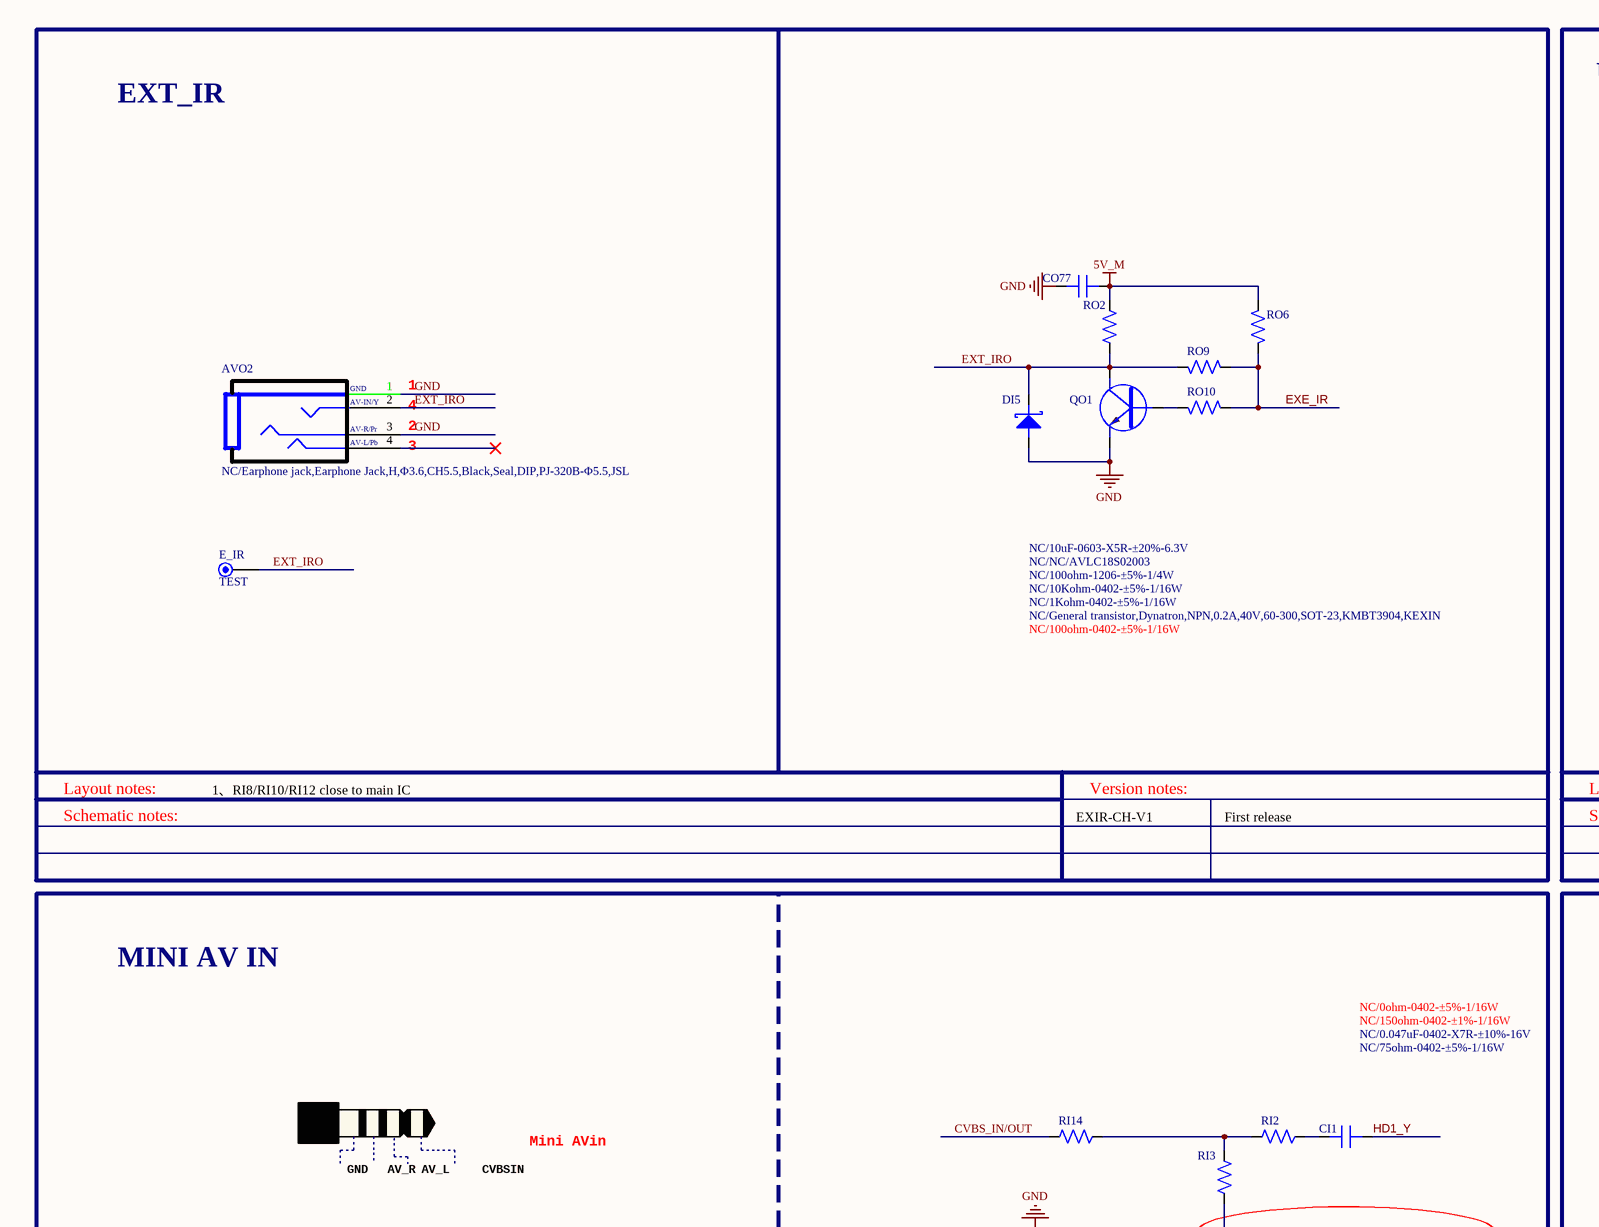
[diagram p0: MISC86383-13.SchDoc, top left]
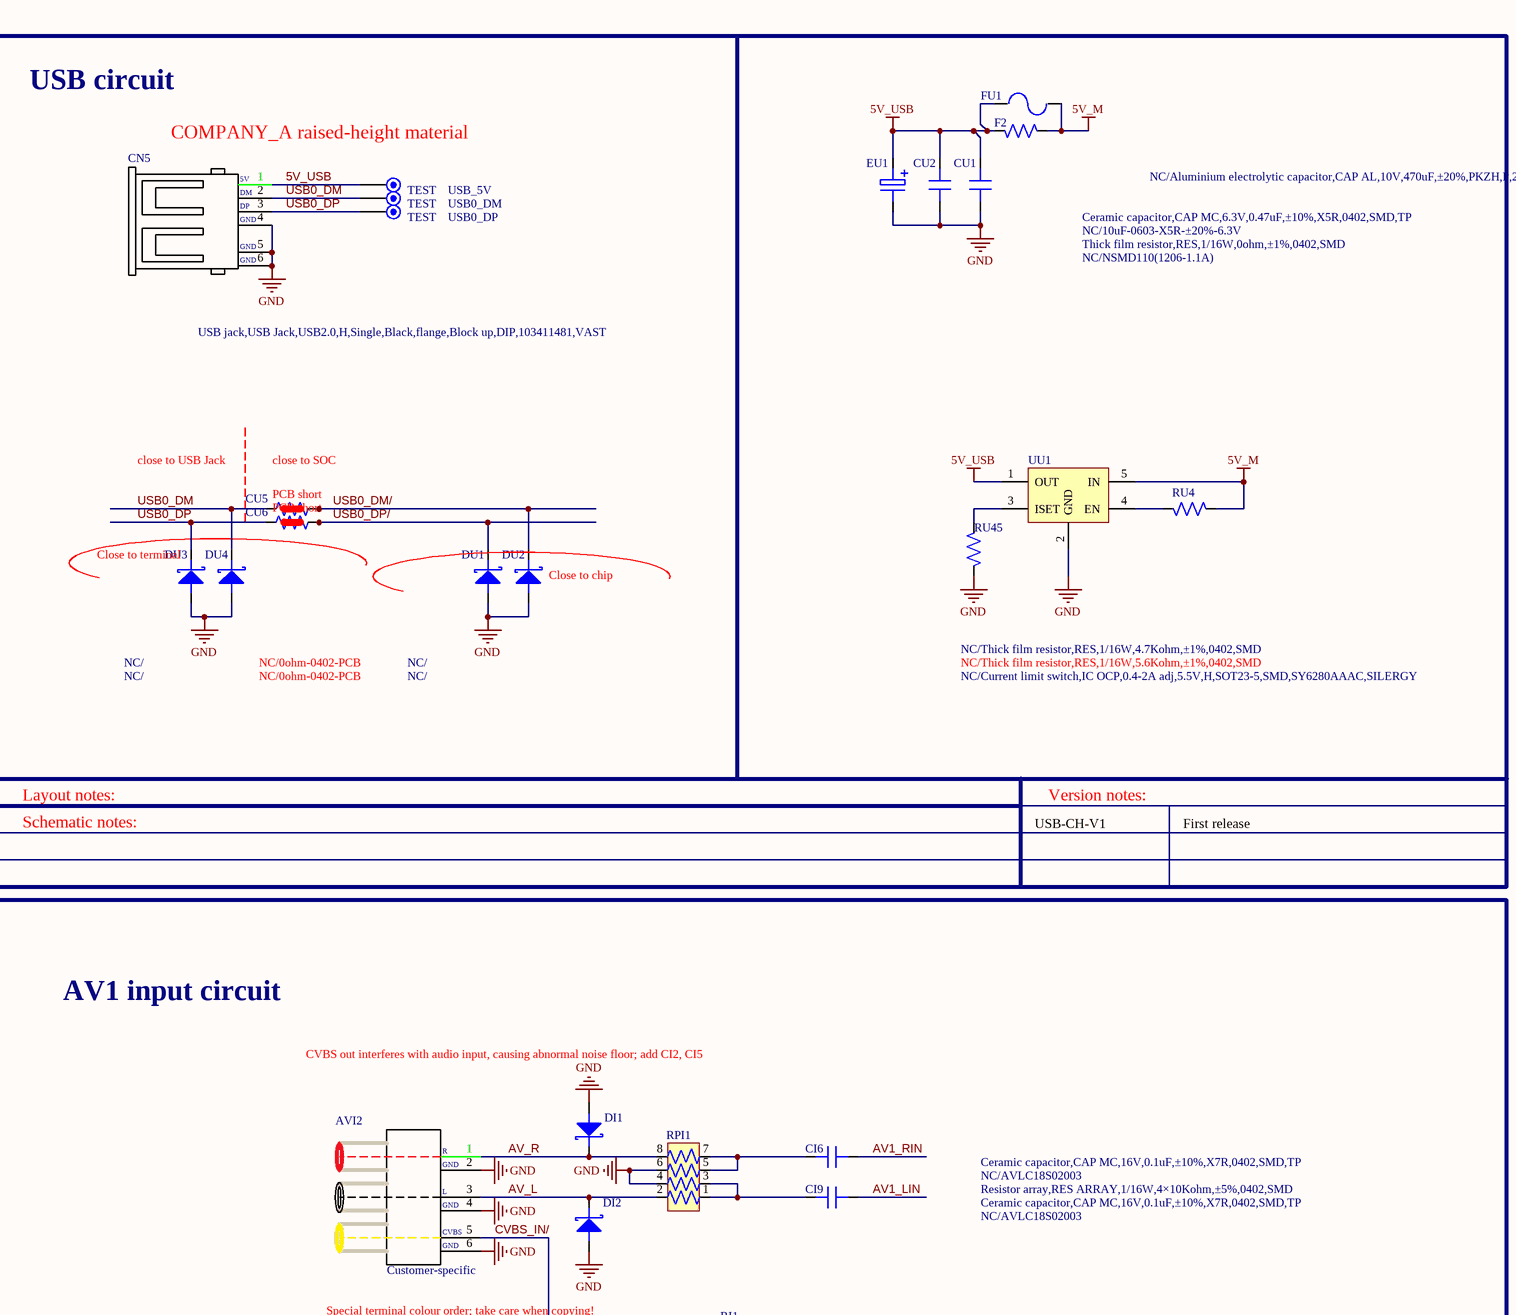
[diagram p1: MISC86383-13.SchDoc, top right]
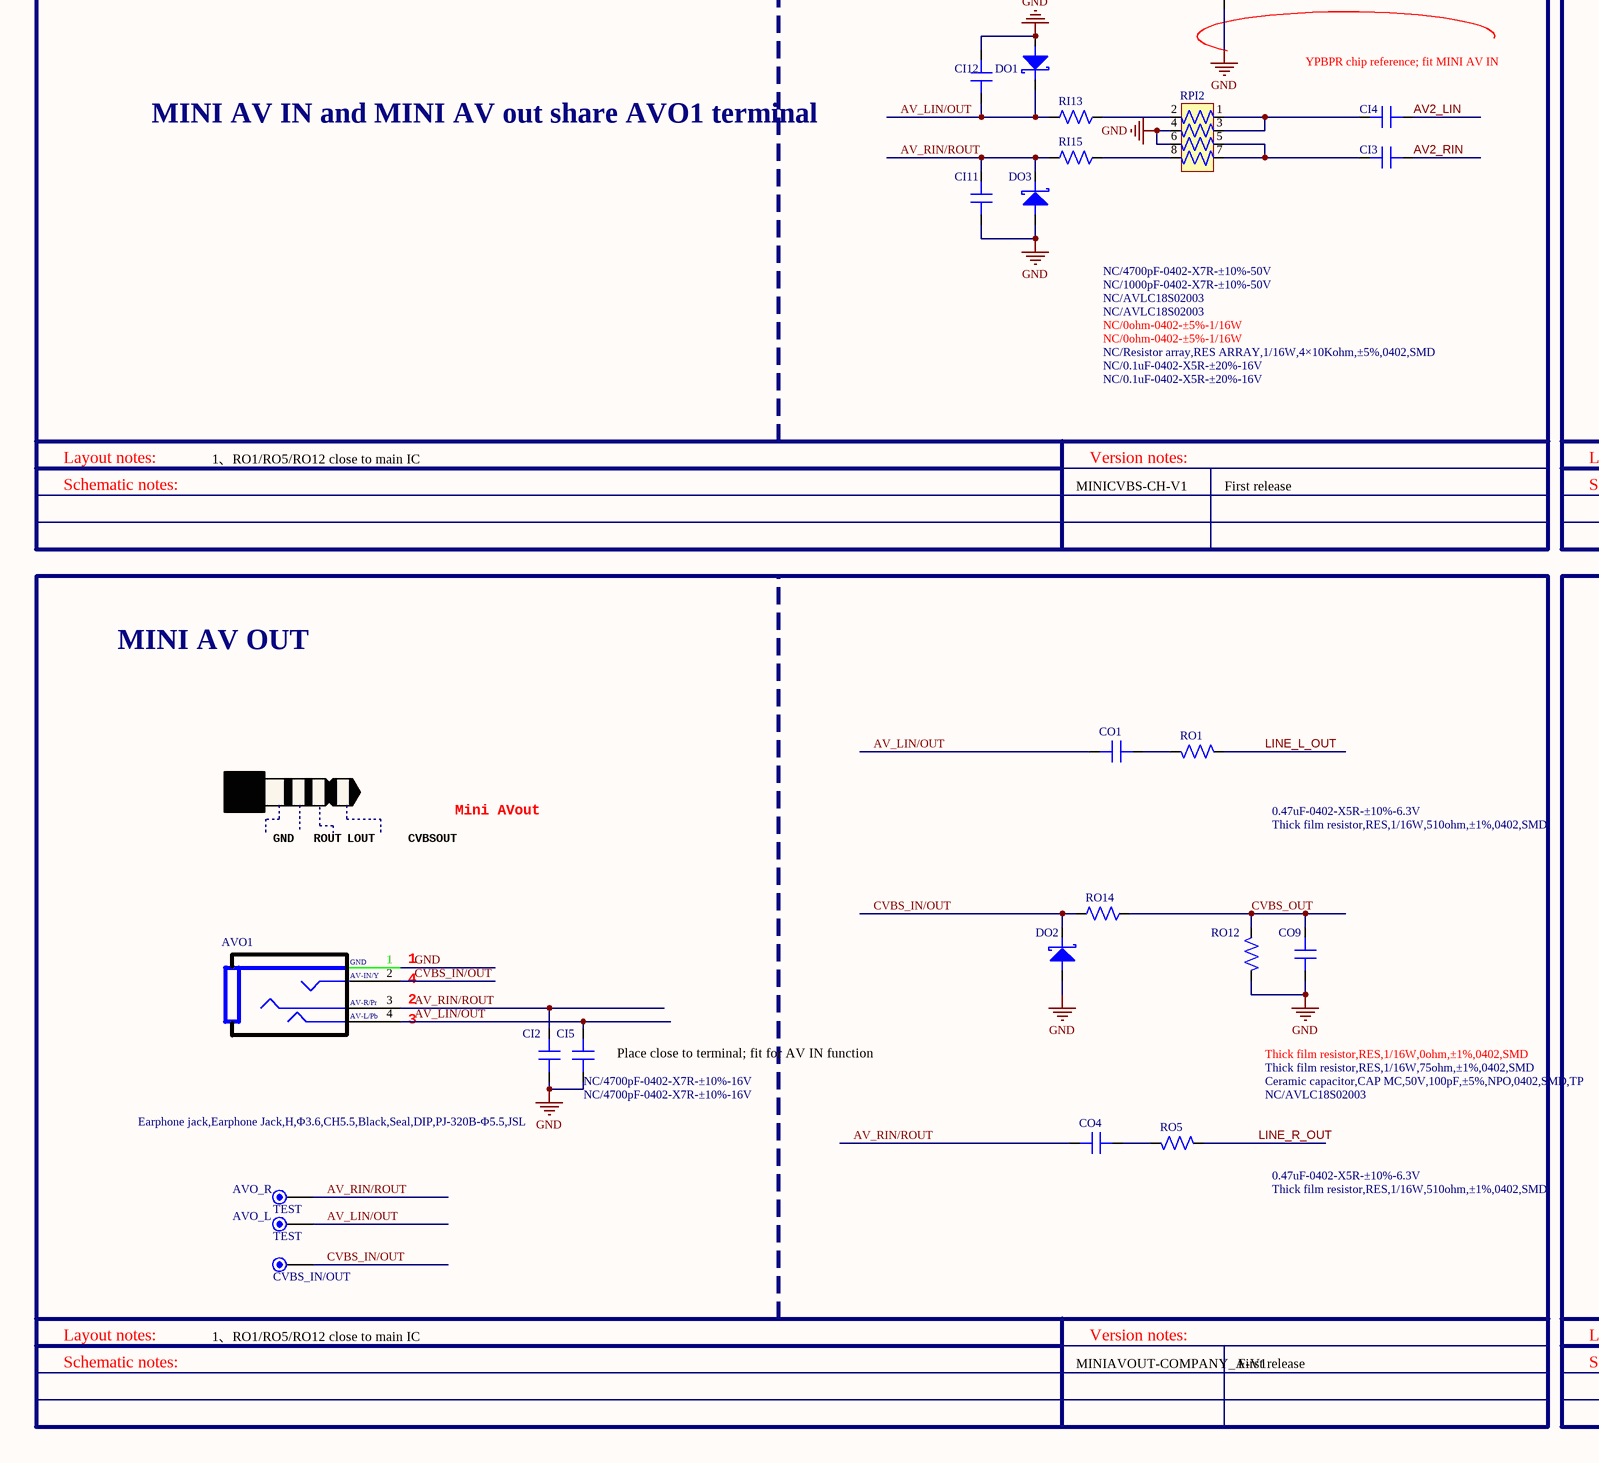
[diagram p2: MISC86383-13.SchDoc, bottom left]
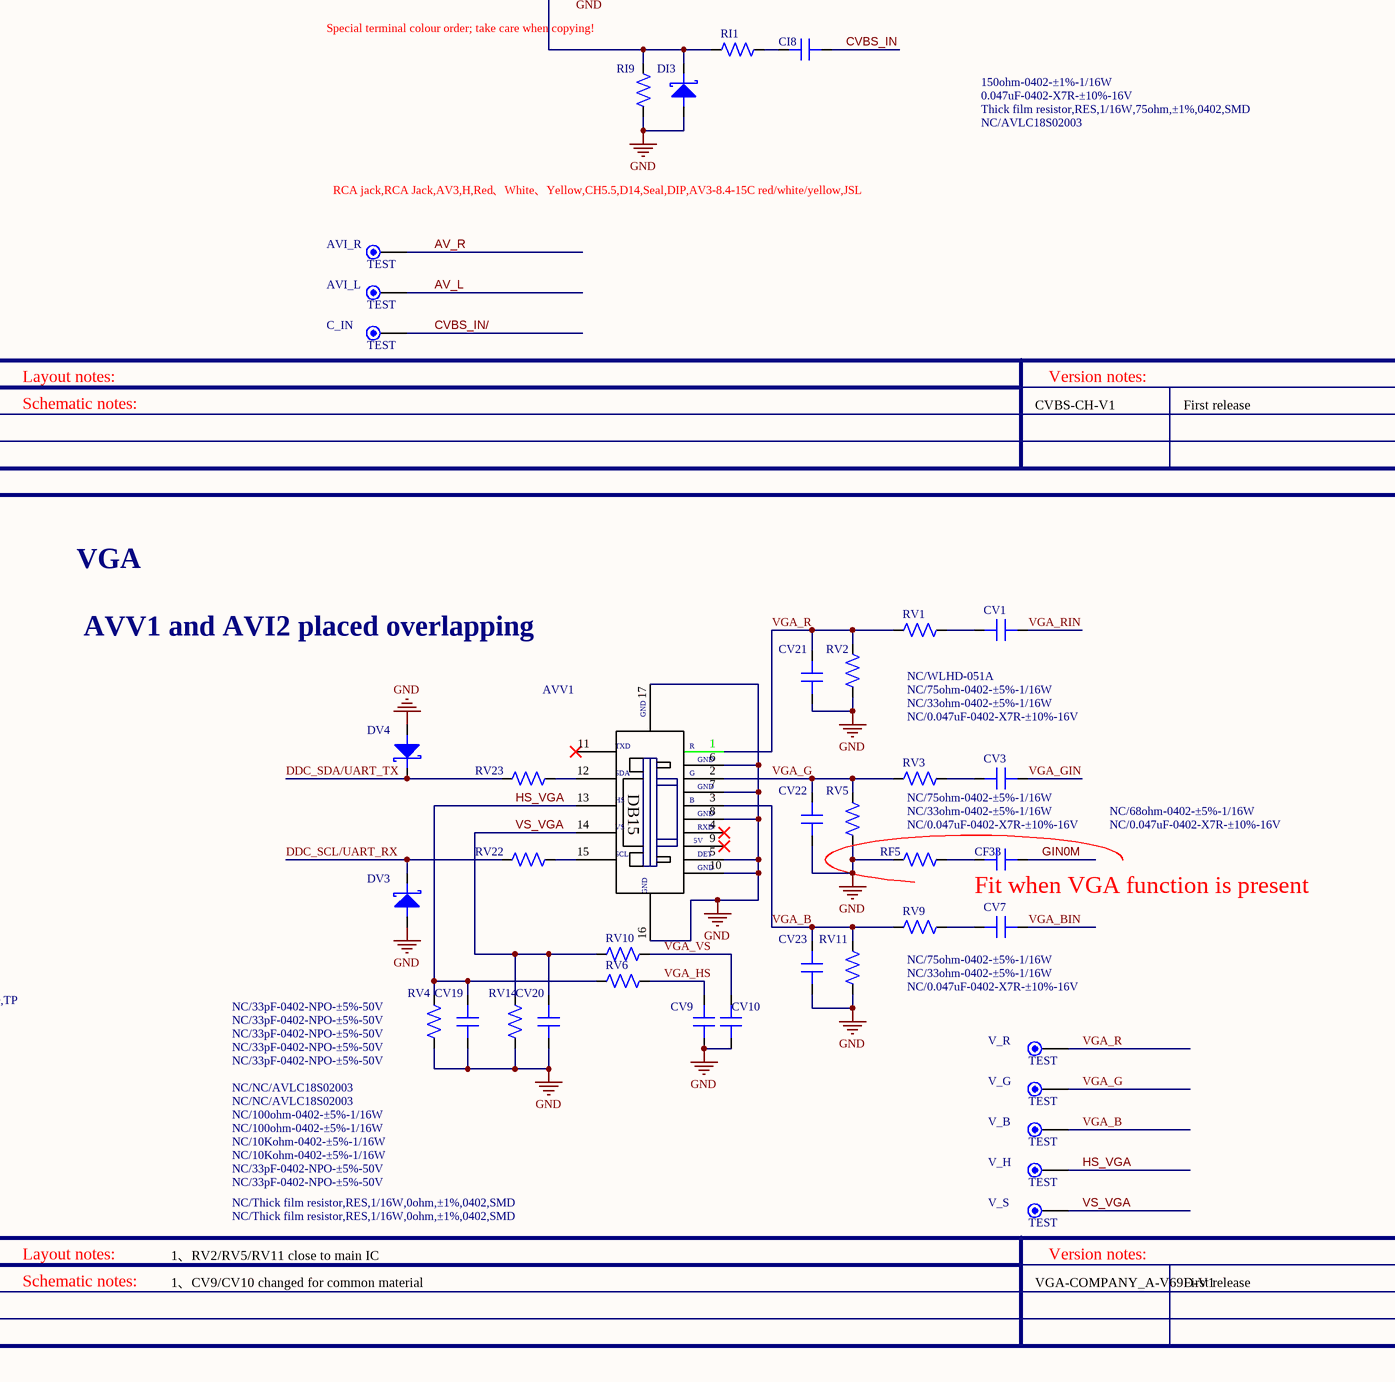
[diagram p3: MISC86383-13.SchDoc, bottom right]
# Altium project MISC86383-33.PrjPCB (part 3 of 8)

## Sheet MISC86383-13.SchDoc
size 609 x 546 mm

### Parts
AVI2  RCA jack,RCA Jack,AV3,H,Red、White、Yellow,CH5.5,D14,Seal,DIP,AV3-8.4-15C red/white/yellow,JSL  [AV3-H14-15]
AVI_L  TEST  [TP]
AVI_R  TEST  [TP]
AVO1  Earphone jack,Earphone Jack,H,Φ3.6,CH5.5,Black,Seal,DIP,PJ-320B-Φ5.5,JSL  [PHONE-HD-43]
AVO2  NC/Earphone jack,Earphone Jack,H,Φ3.6,CH5.5,Black,Seal,DIP,PJ-320B-Φ5.5,JSL  [PHONE-HD-43]
AVO_L  TEST  [TP]
AVO_R  TEST  [TP]
AVV1  NC/WLHD-051A  [DB15-HF-1]
C_IN  TEST  [TP]
CF33  NC/0.047uF-0402-X7R-±10%-16V  [C0402]
CI1  NC/0.047uF-0402-X7R-±10%-16V  [C0402]
CI2  NC/4700pF-0402-X7R-±10%-16V  [C0402]
CI3  NC/0.1uF-0402-X5R-±20%-16V  [C0402]
CI4  NC/0.1uF-0402-X5R-±20%-16V  [C0402]
CI5  NC/4700pF-0402-X7R-±10%-16V  [C0402]
CI6  Ceramic capacitor,CAP MC,16V,0.1uF,±10%,X7R,0402,SMD,TP  [C0402]
CI8  0.047uF-0402-X7R-±10%-16V  [C0402]
CI9  Ceramic capacitor,CAP MC,16V,0.1uF,±10%,X7R,0402,SMD,TP  [C0402]
CI11  NC/1000pF-0402-X7R-±10%-50V  [C0402]
CI12  NC/4700pF-0402-X7R-±10%-50V  [C0402]
CN5  USB jack,USB Jack,USB2.0,H,Single,Black,flange,Block up,DIP,103411481,VAST  [USB-HD-30]
CO1  0.47uF-0402-X5R-±10%-6.3V  [C0402]
CO4  0.47uF-0402-X5R-±10%-6.3V  [C0402]
CO9  Ceramic capacitor,CAP MC,50V,100pF,±5%,NPO,0402,SMD,TP  [C0402]
CO77  NC/10uF-0603-X5R-±20%-6.3V  [C0603]
CU1  NC/10uF-0603-X5R-±20%-6.3V  [C0603]
CU2  Ceramic capacitor,CAP MC,6.3V,0.47uF,±10%,X5R,0402,SMD,TP  [C0402]
CU5  NC/0ohm-0402-PCB  [R0402SC]
CU6  NC/0ohm-0402-PCB  [R0402SC]
CV1  NC/0.047uF-0402-X7R-±10%-16V  [C0402]
CV3  NC/0.047uF-0402-X7R-±10%-16V  [C0402]
CV7  NC/0.047uF-0402-X7R-±10%-16V  [C0402]
CV9  NC/33pF-0402-NPO-±5%-50V  [C0402]
CV10  NC/33pF-0402-NPO-±5%-50V  [C0402]
CV19  NC/33pF-0402-NPO-±5%-50V  [C0402]
CV20  NC/33pF-0402-NPO-±5%-50V  [C0402]
CV21  NC/33pF-0402-NPO-±5%-50V  [C0402]
CV22  NC/33pF-0402-NPO-±5%-50V  [C0402]
CV23  NC/33pF-0402-NPO-±5%-50V  [C0402]
CVBS_IN/OUT  TEST  [TP]  (value not drawn)
DI1  NC/AVLC18S02003  [DIODE-S0402]
DI2  NC/AVLC18S02003  [DIODE-S0402]
DI3  NC/AVLC18S02003  [DIODE-S0402]
DI5  NC/NC/AVLC18S02003  [DIODE-S0402]
DO1  NC/AVLC18S02003  [DIODE-S0402]
DO2  NC/AVLC18S02003  [DIODE-S0402]
DO3  NC/AVLC18S02003  [DIODE-S0402]
DU1  NC/  [DIODE-S0402]
DU2  NC/  [DIODE-S0402]
DU3  NC/  [DIODE-S0402]
DU4  NC/  [DIODE-S0402]
DV3  NC/NC/AVLC18S02003  [DIODE-S0402]
DV4  NC/NC/AVLC18S02003  [DIODE-S0402]
E_IR  TEST  [TP]
EU1  NC/Aluminium electrolytic capacitor,CAP AL,10V,470uF,±20%,PKZH,P,2.5mm,6.3×11,DIP,TP,Koshin  [EC(6.3*11)-V-2.5]
F2  Thick film resistor,RES,1/16W,0ohm,±1%,0402,SMD  [R0402]
FU1  NC/NSMD110(1206-1.1A)  [FUSE1.1A-S]
QO1  NC/General transistor,Dynatron,NPN,0.2A,40V,60-300,SOT-23,KMBT3904,KEXIN  [SOT-23]
RF5  NC/68ohm-0402-±5%-1/16W  [R0402]
RI1  150ohm-0402-±1%-1/16W  [R0402]
RI2  NC/150ohm-0402-±1%-1/16W  [R0402]
RI3  NC/75ohm-0402-±5%-1/16W  [R0402]
RI9  Thick film resistor,RES,1/16W,75ohm,±1%,0402,SMD  [R0402]
RI13  NC/0ohm-0402-±5%-1/16W  [R0402]
RI14  NC/0ohm-0402-±5%-1/16W  [R0402]
RI15  NC/0ohm-0402-±5%-1/16W  [R0402]
RO1  Thick film resistor,RES,1/16W,510ohm,±1%,0402,SMD  [R0402]
RO2  NC/100ohm-1206-±5%-1/4W  [R1206]
RO5  Thick film resistor,RES,1/16W,510ohm,±1%,0402,SMD  [R0402]
RO6  NC/10Kohm-0402-±5%-1/16W  [R0402]
RO9  NC/100ohm-0402-±5%-1/16W  [R0402]
RO10  NC/1Kohm-0402-±5%-1/16W  [R0402]
RO12  Thick film resistor,RES,1/16W,75ohm,±1%,0402,SMD  [R0402]
RO14  Thick film resistor,RES,1/16W,0ohm,±1%,0402,SMD  [R0402]
RPI1  Resistor array,RES ARRAY,1/16W,4×10Kohm,±5%,0402,SMD  [RA0402]
RPI2  NC/Resistor array,RES ARRAY,1/16W,4×10Kohm,±5%,0402,SMD  [RA0402]
RU4  NC/Thick film resistor,RES,1/16W,4.7Kohm,±1%,0402,SMD  [R0402]
RU45  NC/Thick film resistor,RES,1/16W,5.6Kohm,±1%,0402,SMD  [R0402]
RV1  NC/33ohm-0402-±5%-1/16W  [R0402]
RV2  NC/75ohm-0402-±5%-1/16W  [R0402]
RV3  NC/33ohm-0402-±5%-1/16W  [R0402]
RV4  NC/10Kohm-0402-±5%-1/16W  [R0402]
RV5  NC/75ohm-0402-±5%-1/16W  [R0402]
RV6  NC/100ohm-0402-±5%-1/16W  [R0402]
RV9  NC/33ohm-0402-±5%-1/16W  [R0402]
RV10  NC/100ohm-0402-±5%-1/16W  [R0402]
RV11  NC/75ohm-0402-±5%-1/16W  [R0402]
RV14  NC/10Kohm-0402-±5%-1/16W  [R0402]
RV22  NC/Thick film resistor,RES,1/16W,0ohm,±1%,0402,SMD  [R0402]
RV23  NC/Thick film resistor,RES,1/16W,0ohm,±1%,0402,SMD  [R0402]
USB0_DM  TEST  [TP]
USB0_DP  TEST  [TP]
USB_5V  TEST  [TP]
UU1  NC/Current limit switch,IC OCP,0.4-2A adj,5.5V,H,SOT23-5,SMD,SY6280AAAC,SILERGY  [SOP23-5-1]
V_B  TEST  [TP]
V_G  TEST  [TP]
V_H  TEST  [TP]
V_R  TEST  [TP]
V_S  TEST  [TP]

### Blocks framed on the sheet
EXT_IR: AVO2 CO77 DI5 E_IR QO1 RO2 RO6 RO9 RO10
USB circuit: CN5 CU1 CU2 CU5 CU6 DU1-DU4 EU1 F2 FU1 RU4 RU45 USB0_DM USB0_DP USB_5V UU1
AV1 input circuit: AVI2 AVI_L AVI_R C_IN CI6 CI8 CI9 DI1-DI3 RI1 RI9 RPI1
MINI AV OUT: AVO1 AVO_L AVO_R CI2 CI5 CO1 CO4 CO9 CVBS_IN/OUT DO2 RO1 RO5 RO12 RO14

### Nets
5V_M: CO77.1 F2.1 FU1.2 RO2.2 RO6.1 RU4.2 UU1.5(IN)
5V_USB: CN5.1 CU1.2 CU2.1 EU1.1 F2.2 FU1.1 USB_5V.1 UU1.1(OUT)
GND: AVI2.2(GND) AVI2.4(GND) AVI2.6(GND) AVO1.1 AVO2.1 AVO2.3 AVV1.5 AVV1.6(GND) AVV1.7(GND) AVV1.8(GND) AVV1.10(GND) AVV1.16(Shell) AVV1.17(Shell) CI2.1 CI5.1 CI11.2 CI12.2 CN5.4 CN5.5 CN5.6 CO9.1 CO77.2 CU1.1 CU2.2 CV9.1 CV10.1 CV19.1 CV20.1 CV21.1 CV22.1 CV23.1 DI1.A DI2.A DI3.A DI5.A DO1.A DO2.A DO3.A DU1.A DU2.A DU3.A DU4.A DV3.A DV4.A EU1.2 QO1.E RF5.2 RI3.1 RI9.1 RO12.2 RPI1.4 RPI1.6 RPI2.4 RPI2.6 RU45.2 RV2.1 RV4.2 RV5.1 RV11.1 RV14.2 UU1.2(GND)
AV1_LIN: CI9.1
AV1_RIN: CI6.1
AV2_LIN: CI4.1
AV2_RIN: CI3.1
AV_L: AVI2.3(Rin) AVI_L.1 DI2.K RPI1.2
AV_LIN/OUT: AVO1.4 AVO_L.1 CI5.2 CI12.1 CO1.1 DO1.K RI13.1
AV_R: AVI2.1(Lin) AVI_R.1 DI1.K RPI1.8
AV_RIN/ROUT: AVO1.3 AVO_R.1 CI2.2 CI11.1 CO4.1 DO3.K RI15.1
CVBS_IN: CI8.1
CVBS_IN/: AVI2.5(CVBS) C_IN.1 DI3.K RI1.1 RI9.2
CVBS_IN/OUT: AVO1.2 CVBS_IN/OUT.1 DO2.K RI14.1 RO14.1
CVBS_OUT: CO9.2 RO12.1 RO14.2
DDC_SCL/UART_RX: DV3.K RV22.1
DDC_SDA/UART_TX: DV4.K RV23.1
EXE_IR: RO6.2 RO9.2 RO10.2
EXT_IRO: AVO2.2 DI5.K E_IR.1 QO1.C RO2.1 RO9.1
GIN0M: CF33.1
HD1_Y: CI1.1
HS_VGA: AVV1.13(HS) CV19.2 RV4.1 RV6.1 V_H.1
LINE_L_OUT: RO1.1
LINE_R_OUT: RO5.1
USB0_DM: CN5.2 CU5.1 DU4.K USB0_DM.1
USB0_DM/: CU5.2 CU5.3 DU2.K
USB0_DP: CN5.3 CU6.1 DU3.K USB0_DP.1
USB0_DP/: CU6.2 CU6.3 DU1.K
VGA_B: AVV1.3(B) CV23.2 RV9.2 RV11.2 V_B.1
VGA_BIN: CV7.1
VGA_G: AVV1.2(G) CV22.2 RV3.2 RV5.2 V_G.1
VGA_GIN: CV3.1
VGA_HS: CV9.2 RV6.2
VGA_R: AVV1.1(R) CV21.2 RV1.2 RV2.2 V_R.1
VGA_RIN: CV1.1
VGA_VS: CV10.2 RV10.2
VS_VGA: AVV1.14(VS) CV20.2 RV10.1 RV14.1 V_S.1
NetAVV1_12: AVV1.12(SDA) RV23.2
NetAVV1_15: AVV1.15(SCL) RV22.2
NetCF33_2: CF33.2 RF5.1
NetCI1_2: CI1.2 RI2.2
NetCI3_2: CI3.2 RPI2.5 RPI2.7
NetCI4_2: CI4.2 RPI2.1 RPI2.3
NetCI6_2: CI6.2 RPI1.5 RPI1.7
NetCI8_2: CI8.2 RI1.2
NetCI9_2: CI9.2 RPI1.1 RPI1.3
NetCO1_2: CO1.2 RO1.2
NetCO4_2: CO4.2 RO5.2
NetCV1_2: CV1.2 RV1.1
NetCV3_2: CV3.2 RV3.1
NetCV7_2: CV7.2 RV9.1
NetQO1_B: QO1.B RO10.1
NetRI2_1: RI2.1 RI3.2 RI14.2
NetRI13_2: RI13.2 RPI2.2
NetRI15_2: RI15.2 RPI2.8
NetRU4_1: RU4.1 UU1.4(EN)
NetRU45_1: RU45.1 UU1.3(ISET)

Not connected (* = marked no-connect by the designer): AVO2 4*; AVV1 4(NC)* 9(NC)* 11(NC)*

### Notes on the sheet
- COMPANY_A raised-height material
- (near AVO2) 2
- (near AVO2) 4
- (near AVO2) 1
- (near AVO2) 3
- close to USB Jack
- close to SOC
- (near DU3) Close to terminal
- (near DU2) Close to chip
- Layout notes:
- Schematic notes:
- 1、RI8/RI10/RI12 close to main IC
- EXIR-CH-V1
- Version notes:
- First release
- USB-CH-V1
- MINI AV IN
- (near DI1) CVBS out interferes with audio input, causing abnormal noise floor; add CI2, CI5
- GND
- AV_R
- AV_L
- CVBSIN
- Mini AVin
- (near CI4) YPBPR chip reference; fit MINI AV IN
- Special terminal colour order; take care when copying!
- MINI AV IN and MINI AV out share AVO1 terminal
- 1、RO1/RO5/RO12 close to main IC
- MINICVBS-CH-V1
- CVBS-CH-V1
- VGA
- AVV1 and AVI2 placed overlapping
- ROUT
- LOUT
- CVBSOUT
- Mini AVout
- (near AVO1) 4
- (near AVO1) 1
- (near CF33) Fit when VGA function is present
- (near AVO1) 2
- (near AVO1) 3
- (near CI5) Place close to terminal; fit for AV IN function
- MINIAVOUT-COMPANY_A-V1
- 1、RV2/RV5/RV11 close to main IC
- 1、CV9/CV10 changed for common material
- VGA-COMPANY_A-V69D-V1
- (near V_S) Version notes:

### Library data of the parts
AVI2 = XXX.XXX.0003577-DLMI: RCA jack,RCA Jack,AV3,H,Red、White、Yellow,CH5.5,D14,Seal,DIP,RC075-F03L3BY-L,YUQIU-DLMI
AVO1 AVO2 = 耳机端子,Earphone Jack,H,Φ3.6,CH5.5,Black,DIP-DLMI
AVV1 = WLHD-051A-DLMI-DB15: CN-DB15-horizontal-#-#-#
CF33 CI1 CI8 CV1 CV3 CV7 = 0.047uF-0402-X7R-±10%-16V-D
CI2 CI5 CO9 = 100pF-0402-NPO-±5%-50V-D
CI3 CI4 CI6 CI9 CU2 = 0.1uF-0402-Y5V-+80%-20%-16V-D
CI11 CI12 = 1000pF-0402-X7R-±10%-50V-D
CN5 = PKG-003212/P000071027: USB jack,USB2.0,H,Single,Block up,DIP,U250FD004S1549BY-DLMI
CO1 CO4 = 1uF-0402-X5R-±20%-6.3V-D
CO77 CU1 = 10uF-0603-X5R-±20%-6.3V-D
CU5 CU6 = 0ohm-0402-PCB-D
CV9 CV10 CV19-CV23 = 30pF-0402-NPO-±5%-50V-D
DI1-DI3 DI5 DO1-DO3 DU1-DU4 DV3 DV4 = AVLC18S02003-D
EU1 = 470uF-10V-±20%-6.3×11-105℃-黑底白字-编带-F=2.5-XF-DHAI: Electrolytic
F2 = 5R1ohm-0402-±5%-1/16W-D
FU1 = 004.026.0000039-D: Self-resetting fuse,FUSE PTC,1.1A,6V,1206,SMD,TP,TLC-D
QO1 = LMBT3904LT1G-D-NPN: Q-NPN-#-#-#
RF5 = 68ohm-0402-±5%-1/16W-D
RI1 RI2 = 150ohm-0402-±1%-1/16W-D
RI3 RI9 RO12 RV2 RV5 RV11 = 75ohm-0402-±5%-1/16W-D
RI13-RI15 RO14 = 0ohm-0402-±5%-1/16W-D
RO1 RO5 = 510ohm-0402-±5%-1/16W-D
RO2 = 100ohm-1206-±5%-1/4W-D: RES
RO6 RV4 RV14 = 10Kohm-0402-±5%-1/16W-D
RO9 RV6 RV10 RV22 RV23 = 100ohm-0402-±5%-1/16W-D
RO10 = 1Kohm-0402-±5%-1/16W-D
RPI1 RPI2 = 4*100ohm-0402-±5%-1/16W-D
RU4 = 4K7ohm-0402-±5%-1/16W-D
RU45 = 4K7ohm-0402-±1%-1/16W-D
RV1 RV3 RV9 = 33ohm-0402-±5%-1/16W-D
UU1 = 004.010.0000334-D: Current limit switch,IC OCP,0.4-2A adj,5.5V,H,SOT23-5,SMD,SY6280AAAC,SILERGY-D